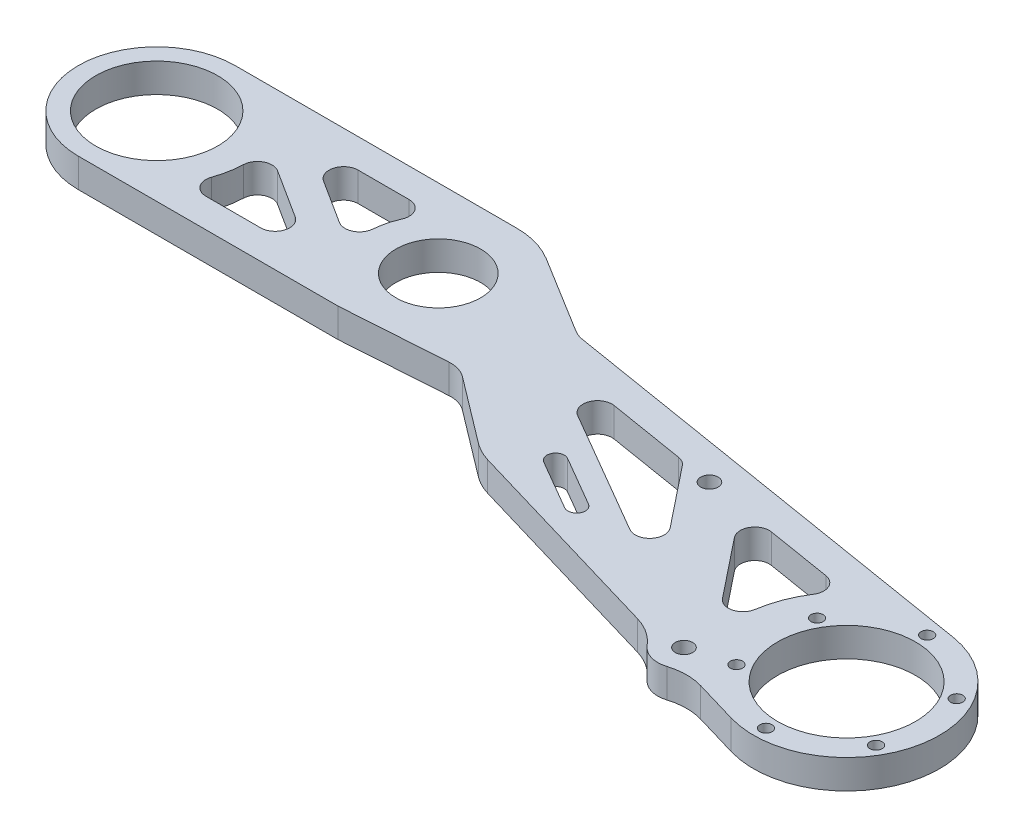
from build123d import *

# Parameters (mm, degrees)
SKETCH_1_R          = 21
SKETCH_1_R_2        = 14.575
SKETCH_1_R_3        = 23.75
SKETCH_1_R_4        = 2.1
SKETCH_1_R_5        = 3
EXTRUDE_1_DEPTH     = 10
CUT_EXTRUDE_1_DEPTH = 10
FILLET_1_R          = 20
CUT_EXTRUDE_2_DEPTH = 10
FILLET_2_R          = 5
SKETCH_5_R          = 3
CUT_EXTRUDE_3_DEPTH = 10
CUT_EXTRUDE_5_DEPTH = 10


with BuildPart() as part:
    # 草图1 → 凸台-拉伸1 (new body)
    with BuildSketch(Plane(origin=(0, 0, 0), x_dir=(1, 0, 0), z_dir=(0, 1, 0))):
        with BuildLine():
            Line((0, 27), (96.94985335, 27))
            ThreePointArc((96.94985335, 27), (104.319003455, 25.974903787), (111.128591496, 22.977453832))
            Line((111.128591496, 22.977453832), (137.853241587, 6.486426651))
            ThreePointArc((137.853241587, 6.486426651), (139.604326734, 5.629209592), (141.488462469, 5.12805811))
            Line((141.488462469, 5.12805811), (294.137288277, -19.871137584))
            ThreePointArc((294.137288277, -19.871137584), (320.161534926, -58.578669293), (279.908528522, -82.141986125))
            Line((279.908528522, -82.141986125), (257.295172569, -75.46881036))
            ThreePointArc((257.295172569, -75.46881036), (248.237976105, -77.886212941), (241.944328029, -70.938793499))
            Line((241.944328029, -70.938793499), (95.820417973, -27.817792917))
            ThreePointArc((95.820417973, -27.817792917), (93.01947824, -27.205504027), (90.159770359, -27))
            Line((90.159770359, -27), (0, -27))
            ThreePointArc((0, -27), (-27, 0), (0, 27))
        make_face()
        with Locations(Location((0, 0, 0), (0, 0, 270))):
            Circle(SKETCH_1_R, mode=Mode.SUBTRACT)
        with Locations(Location((96.94985335, 0, 0), (0, 0, 270))):
            Circle(SKETCH_1_R_2, mode=Mode.SUBTRACT)
        with Locations(Location((288.965564705, -51.450454792, 0), (0, 0, 270))):
            Circle(SKETCH_1_R_3, mode=Mode.SUBTRACT)
        with Locations(Location((288.965564705, -23.700454792, 0), (0, 0, 270))):
            Circle(SKETCH_1_R_4, mode=Mode.SUBTRACT)
        with Locations(Location((312.99776966, -37.575454792, 0), (0, 0, 270))):
            Circle(SKETCH_1_R_4, mode=Mode.SUBTRACT)
        with Locations(Location((312.99776966, -65.325454792, 0), (0, 0, 270))):
            Circle(SKETCH_1_R_4, mode=Mode.SUBTRACT)
        with Locations(Location((288.965564705, -79.200454792, 0), (0, 0, 270))):
            Circle(SKETCH_1_R_4, mode=Mode.SUBTRACT)
        with Locations(Location((264.93335975, -65.325454792, 0), (0, 0, 270))):
            Circle(SKETCH_1_R_4, mode=Mode.SUBTRACT)
        with Locations(Location((264.93335975, -37.575454792, 0), (0, 0, 270))):
            Circle(SKETCH_1_R_4, mode=Mode.SUBTRACT)
        with Locations(Location((250.785267532, -69.254219754, 0), (0, 0, 270))):
            Circle(SKETCH_1_R_5, mode=Mode.SUBTRACT)
    extrude(amount=EXTRUDE_1_DEPTH)

    # 草图3 → 切除-拉伸1 (cut)
    with BuildSketch(Plane(origin=(0, 10, 0), x_dir=(1, 0, 0), z_dir=(0, 1, 0))):
        with BuildLine():
            Line((243.704770173, -111.253970394), (131.873115991, -26.616980894))
            ThreePointArc((131.873115991, -26.616980894), (128.702921113, -25.009854291), (125.170844375, -24.613085592))
            Line((125.170844375, -24.613085592), (88.824772335, -27.044605234))
            Line((88.824772335, -27.044605234), (243.704770173, -111.253970394))
        make_face()
    extrude(amount=-CUT_EXTRUDE_1_DEPTH, mode=Mode.SUBTRACT)

    # 圆角1
    fillet_1_edges = [part.edges().sort_by_distance(p)[0] for p in [
        (257.295172569, 5, 75.46881036),
        (241.944328029, 5, 70.938793499),
        (157.515855554, 5, 46.024046766),
    ]]
    fillet(fillet_1_edges, radius=FILLET_1_R)

    # 草图4 → 切除-拉伸2 (cut)
    with BuildSketch(Plane(origin=(0, 10, 0), x_dir=(1, 0, 0), z_dir=(0, 1, 0))):
        with BuildLine():
            ThreePointArc((73.530936261, -7.448821877), (73.010770558, 5.554362258), (79.203568528, 17))
            Line((79.203568528, 17), (35.21775864, 17))
            Line((35.21775864, 17), (73.530936261, -7.448821877))
        make_face()
        with BuildLine():
            Line((69.908772681, -17), (29.781319723, 8.606567001))
            ThreePointArc((29.781319723, 8.606567001), (30.653969418, -4.618891526), (25.922962794, -17))
            Line((25.922962794, -17), (69.908772681, -17))
        make_face()
        with BuildLine():
            Line((218.588169342, -17.631723767), (252.130615229, -59.711749917))
            ThreePointArc((252.130615229, -59.711749917), (252.70586007, -40.94824932), (262.247669453, -24.781810782))
            Line((262.247669453, -24.781810782), (218.588169342, -17.631723767))
        make_face()
        Polygon((139.872298853, -4.740478518), (229.34372575, -56.794041123), (195.054934366, -13.777701679), align=None)
    extrude(amount=-CUT_EXTRUDE_2_DEPTH, mode=Mode.SUBTRACT)

    # 圆角2
    fillet_2_edges = [part.edges().sort_by_distance(p)[0] for p in [
        (25.922962794, 5, 17),
        (29.781319723, 5, -8.606567001),
        (69.908772681, 5, 17),
        (139.872298853, 5, 4.740478518),
        (195.054934366, 5, 13.777701679),
        (229.34372575, 5, 56.794041123),
        (262.247669453, 5, 24.781810782),
        (252.130615229, 5, 59.711749917),
        (218.588169342, 5, 17.631723767),
        (79.203568528, 5, -17),
        (73.530936261, 5, 7.448821877),
        (35.21775864, 5, -17),
    ]]
    fillet(fillet_2_edges, radius=FILLET_2_R)

    # 草图5 → 切除-拉伸3 (cut)
    with BuildSketch(Plane(origin=(0, 10, 0), x_dir=(1, 0, 0), z_dir=(0, 1, 0))):
        with Locations(Location((205.845927584, -15.544935392, 0), (0, 0, 270))):
            Circle(SKETCH_5_R)
    extrude(amount=-CUT_EXTRUDE_3_DEPTH, mode=Mode.SUBTRACT)

    # 草图7 → 切除-拉伸5 (cut)
    with BuildSketch(Plane.XZ):
        with BuildLine():
            Line((171.32105295, 38.077089469), (188.608233051, 48.134594337))
            ThreePointArc((188.608233051, 48.134594337), (192.709935796, 47.050143053), (191.625484511, 42.948440307))
            Line((191.625484511, 42.948440307), (174.338304411, 32.890935439))
            ThreePointArc((174.338304411, 32.890935439), (170.236601666, 33.975386724), (171.32105295, 38.077089469))
        make_face()
    extrude(amount=-CUT_EXTRUDE_5_DEPTH, mode=Mode.SUBTRACT)


solid = part.part
